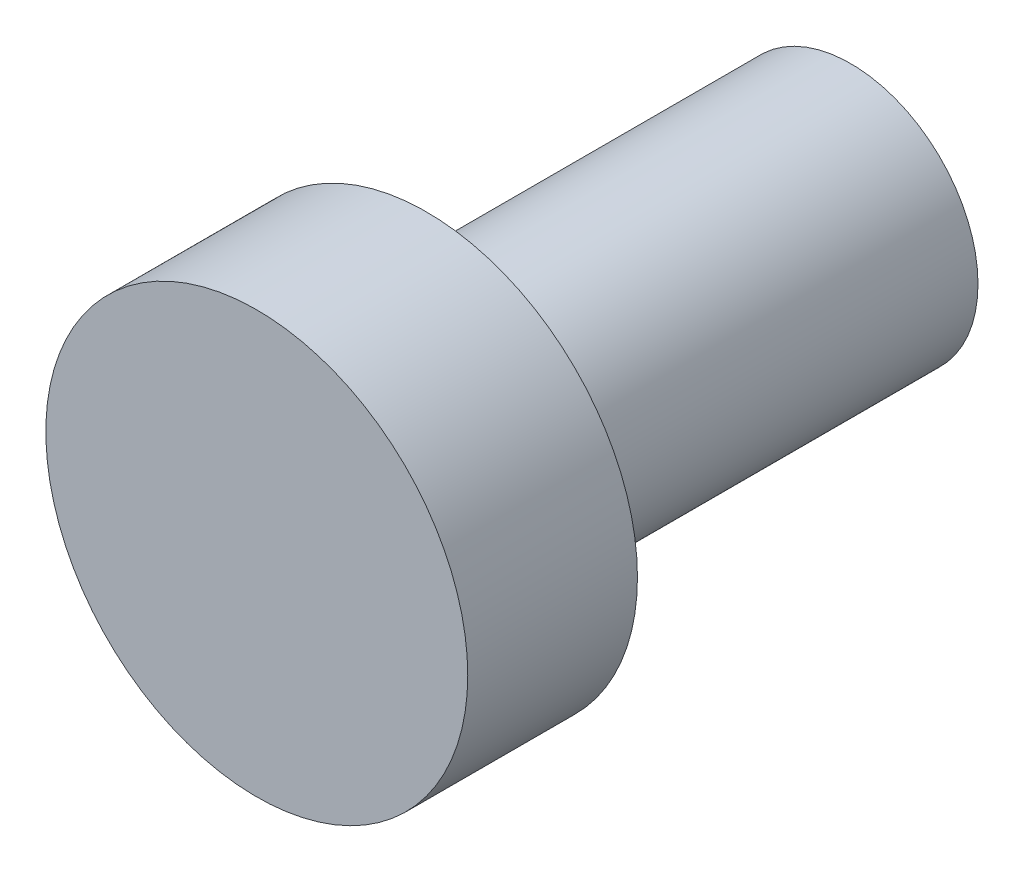
SolidWorks part; units mm, degrees
ref_plane "Front Plane" through (0, 0, 0) normal (0, 0, 1) x (1, 0, 0)
ref_plane "Top Plane" through (0, 0, 0) normal (0, 1, 0) x (1, 0, 0)
ref_plane "Right Plane" through (0, 0, 0) normal (1, 0, 0) x (0, 0, -1)
other "Configuration Table"
sketch "Sketch1" plane through (0, 0, 0) normal (0, 0, 1) x (1, 0, 0)
  circle A1 centre (45.1978, 32.0258) radius 1.5
extrude "Boss-Extrude1" add sketch "Sketch1" against normal blind 5
sketch "Sketch2" plane through (0, 0, 0) normal (0, 0, 1) x (1, 0, 0)
  circle A0 centre (45.1978, 32.0258) radius 2.4864
extrude "Boss-Extrude2" add sketch "Sketch2" along normal blind 2
